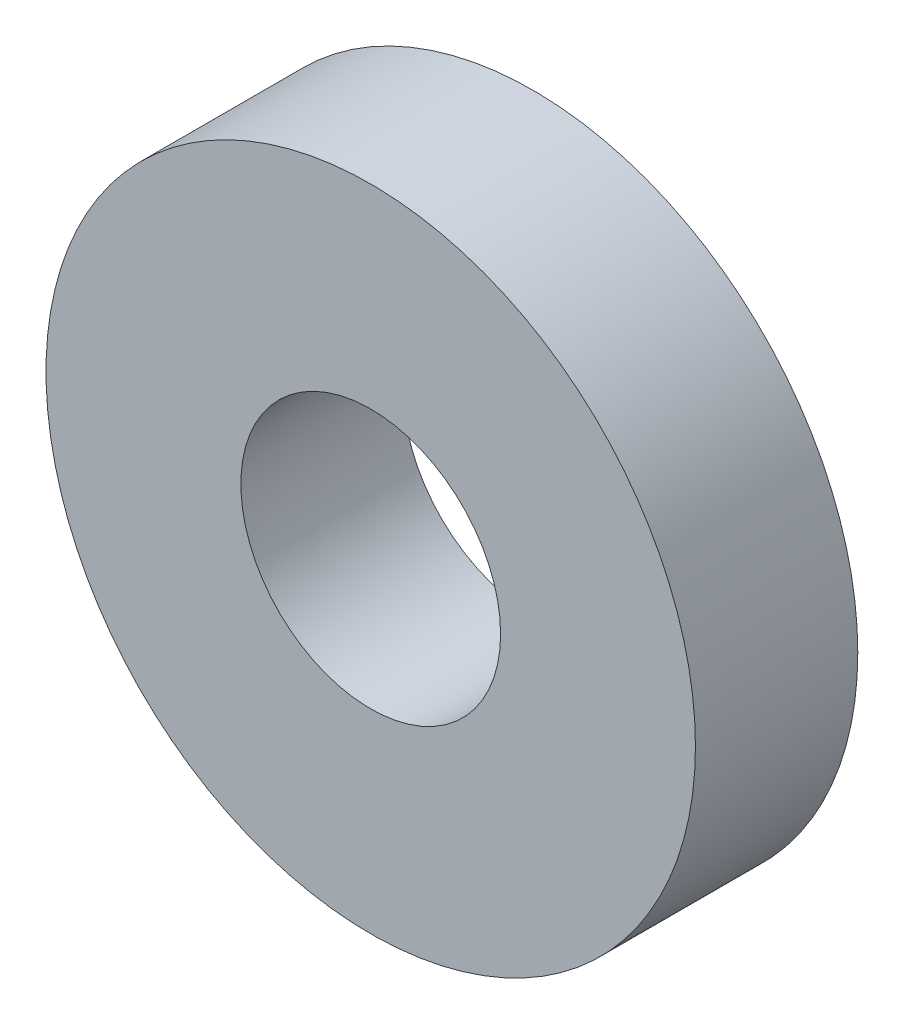
from build123d import *

# Parameters (mm, degrees)
SKETCH1_R           = 4
SKETCH1_R_2         = 1.6
BOSS_EXTRUDE1_DEPTH = 2


with BuildPart() as part:
    # Sketch1 → Boss-Extrude1 (new body)
    with BuildSketch(Plane.XY):
        Circle(SKETCH1_R)
        Circle(SKETCH1_R_2, mode=Mode.SUBTRACT)
    extrude(amount=BOSS_EXTRUDE1_DEPTH)


solid = part.part
